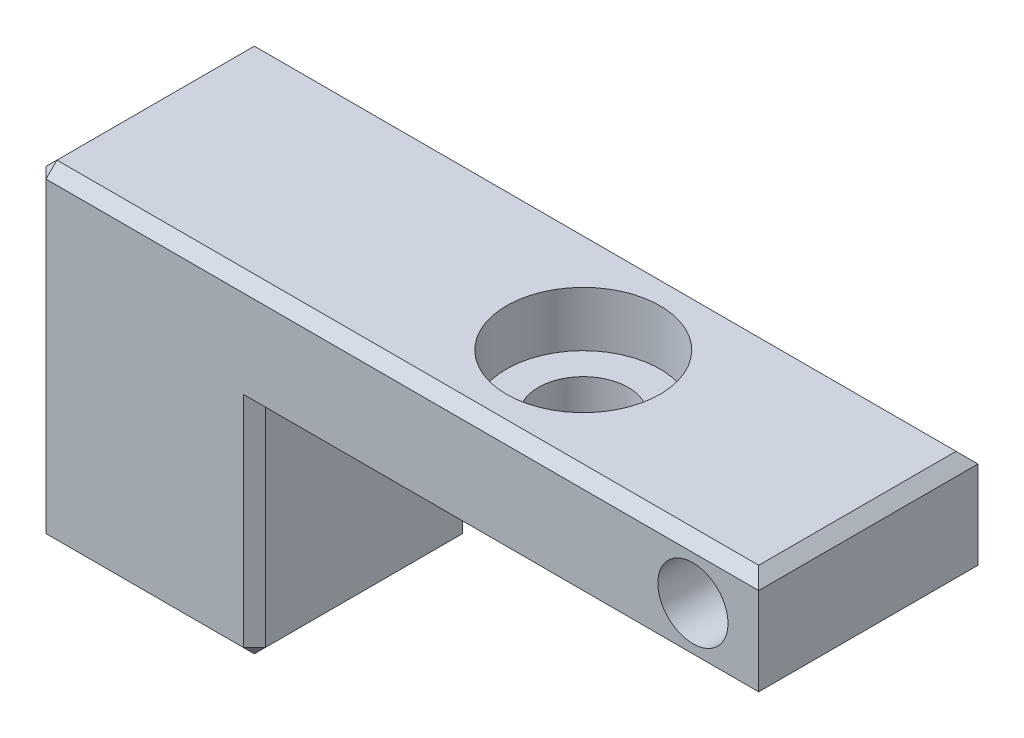
from build123d import *

# Parameters (mm, degrees)
SKETCH1_W             = 33
SKETCH1_H             = 15
BOSS_EXTRUDE1_DEPTH   = 10
SKETCH2_W             = 23
SKETCH2_H             = 10
CUT_EXTRUDE1_DEPTH    = 20
M4_TAPPED_HOLE1_D     = 3.3
M4_TAPPED_HOLE1_DEPTH = 10.1
M4_TAPPED_HOLE1_TIP   = 0.991420021
CHAMFER1_SIZE         = 0.5
SKETCH6_R             = 3.5
CUT_EXTRUDE3_DEPTH    = 2.5
SKETCH7_R             = 1.6
CUT_EXTRUDE4_DEPTH    = 3
SKETCH8_R             = 2.05
CUT_EXTRUDE5_DEPTH    = 10


with BuildPart() as part:
    # Sketch1 → Boss-Extrude1 (new body)
    with BuildSketch(Plane.XY):
        Rectangle(SKETCH1_W, SKETCH1_H)
    extrude(amount=BOSS_EXTRUDE1_DEPTH)

    # Sketch2 → Cut-Extrude1 (cut)
    with BuildSketch(Plane.XY.offset(10)):
        with Locations((5, -2.5)):
            Rectangle(SKETCH2_W, SKETCH2_H)
    extrude(amount=-CUT_EXTRUDE1_DEPTH, mode=Mode.SUBTRACT)

    # M4 Tapped Hole1
    with Locations(Plane(origin=(0, -7.5, 0), x_dir=(-1, 0, 0), z_dir=(0, -1, 0))):
        with Locations((11.5, -5)):
            Hole(M4_TAPPED_HOLE1_D / 2, depth=M4_TAPPED_HOLE1_DEPTH)
            with Locations((0, 0, -(M4_TAPPED_HOLE1_DEPTH + M4_TAPPED_HOLE1_TIP / 2))):  # 118° drill point
                Cone(0, M4_TAPPED_HOLE1_D / 2, M4_TAPPED_HOLE1_TIP, mode=Mode.SUBTRACT)

    # Chamfer1
    chamfer1_edges = [part.edges().sort_by_distance(p)[0] for p in [
        (-16.5, 0, 10),
        (-11.5, -7.5, 10),
        (5, 2.5, 0),
        (-6.5, -2.5, 0),
        (16.5, 2.5, 5),
        (-6.5, -7.5, 5),
        (5, 2.5, 10),
        (-6.5, -2.5, 10),
        (-11.5, -7.5, 0),
        (-16.5, 0, 0),
        (0, 7.5, 0),
        (0, 7.5, 10),
        (-16.5, -7.5, 5),
        (-16.5, 7.5, 5),
        (16.5, 7.5, 5),
    ]]
    chamfer(chamfer1_edges, length=CHAMFER1_SIZE)

    # Sketch6 → Cut-Extrude3 (cut)
    with BuildSketch(Plane(origin=(0, 7.5, 0), x_dir=(1, 0, 0), z_dir=(0, 1, 0))):
        with Locations(Location((3.5, -5, 0), (0, 0, 270))):
            Circle(SKETCH6_R)
    extrude(amount=-CUT_EXTRUDE3_DEPTH, mode=Mode.SUBTRACT)

    # Sketch7 → Cut-Extrude4 (cut)
    with BuildSketch(Plane(origin=(0, 0, 0), x_dir=(-1, 0, 0), z_dir=(0, 0, -1))):
        with Locations((-13.5, 5)):
            Circle(SKETCH7_R)
    cut_extrude4 = extrude(amount=-CUT_EXTRUDE4_DEPTH, mode=Mode.SUBTRACT)

    # Mirror1: Cut-Extrude4 across plane
    add(cut_extrude4.mirror(Plane(origin=(0, 0, 5), x_dir=(1, 0, 0), z_dir=(0, 0, -1))), mode=Mode.SUBTRACT)

    # Sketch8 → Cut-Extrude5 (cut)
    with BuildSketch(Plane(origin=(0, 5, 0), x_dir=(1, 0, 0), z_dir=(0, 1, 0))):
        with Locations(Location((3.5, -5, 0), (0, 0, 270))):
            Circle(SKETCH8_R)
    extrude(amount=-CUT_EXTRUDE5_DEPTH, mode=Mode.SUBTRACT)


solid = part.part
